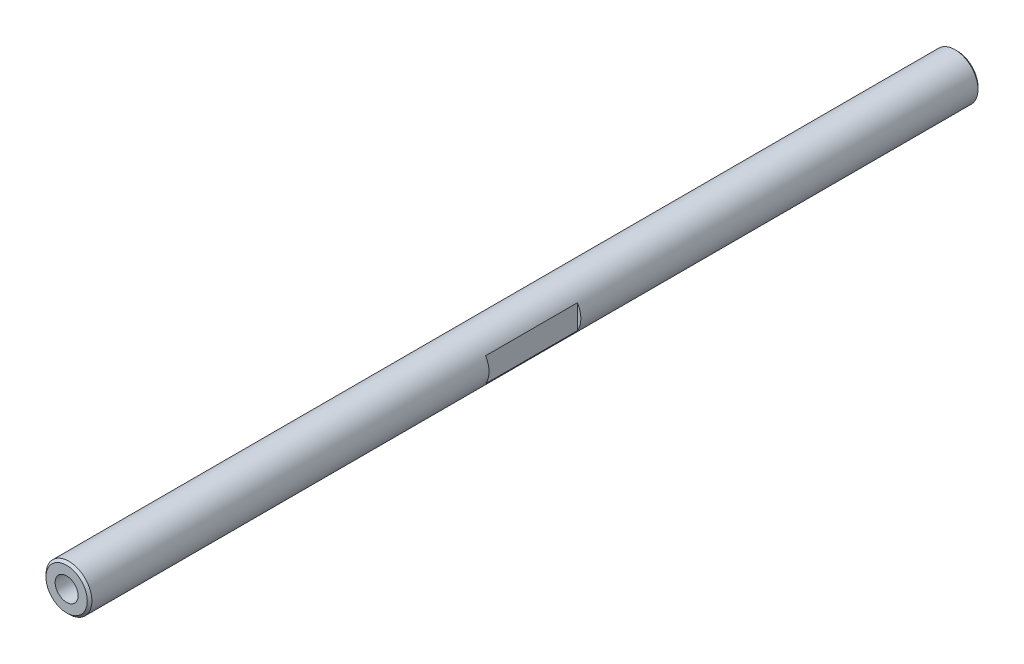
SolidWorks part; units mm, degrees
ref_plane "前视基准面" through (0, 0, 0) normal (0, 0, 1) x (1, 0, 0)
ref_plane "上视基准面" through (0, 0, 0) normal (0, 1, 0) x (1, 0, 0)
ref_plane "右视基准面" through (0, 0, 0) normal (1, 0, 0) x (0, 0, -1)
sketch "草图1" plane through (0, 0, 0) normal (0, 0, 1) x (1, 0, 0)
  circle A0 centre (0, 0) radius 5
  dimension "D1" = 10
extrude "凸台-拉伸1" add sketch "草图1" along normal mid plane 194
sketch "草图2" plane through (0, 0, 0) normal (0, 0, 1) x (1, 0, 0)
  line L0 (-4.25, 2.6339) -> (-4.25, -2.6339)
  line L1 (4.25, 2.6339) -> (4.25, -2.6339)
  line L2 (0, 0) -> (0, 5) construction
  arc A0 (-4.25, 2.6339) -> (-4.25, -2.6339) centre (0, 0) ccw
  circle A1 centre (0, 0) radius 5 construction
  arc A2 (4.25, -2.6339) -> (4.25, 2.6339) centre (0, 0) ccw
  point P1 (0, 5)
  dimension "D1" = 8.5
extrude "切除-拉伸1" cut sketch "草图2" against normal mid plane 20
hole_wizard "M6 螺纹孔1" positions "草图3" profile "草图4" tap size "M6" standard "GB"
sketch "草图3" plane through (0, 0, 97) normal (0, 0, 1) x (1, 0, 0)
  point P0 (0, 0)
sketch "草图4" plane through (0, 0, 97) normal (1, 0, 0) x (0, -1, 0)
  line L0 (0, 0) -> (0, 16.5022)
  line L1 (0, 16.5022) -> (2.5, 15)
  line L2 (2.5, 15) -> (2.5, 0)
  line L5 (2.5, 0) -> (0, 0)
  line L10 (0, 16.5022) -> (-2.5, 15) construction
  line L11 (0, -6.35) -> (0, 107.95) construction
  dimension "螺纹孔钻头直径" = 5
  dimension "螺纹孔钻头深度" = 15
  dimension "导头角度" = 118
cosmetic thread "孔螺蚊线1" parameters "D1"=12, "D2"=6
hole_wizard "M6 螺纹孔2" positions "草图5" profile "草图6" tap size "M6" standard "GB"
sketch "草图5" plane through (0, 0, -97) normal (0, 0, -1) x (-1, 0, 0)
  point P0 (0, 0)
sketch "草图6" plane through (0, 0, -97) normal (1, 0, 0) x (0, 1, 0)
  line L0 (0, 0) -> (0, 16.5022)
  line L1 (0, 16.5022) -> (2.5, 15)
  line L2 (2.5, 15) -> (2.5, 0)
  line L5 (2.5, 0) -> (0, 0)
  line L10 (0, 16.5022) -> (-2.5, 15) construction
  line L11 (0, -6.35) -> (0, 107.95) construction
  dimension "螺纹孔钻头直径" = 5
  dimension "螺纹孔钻头深度" = 15
  dimension "导头角度" = 118
cosmetic thread "孔螺蚊线2" parameters "D1"=12, "D2"=6
chamfer "倒角1" distance 0.5 angle 45 2 edges at (5, 0, 97) (5, 0, -97)
